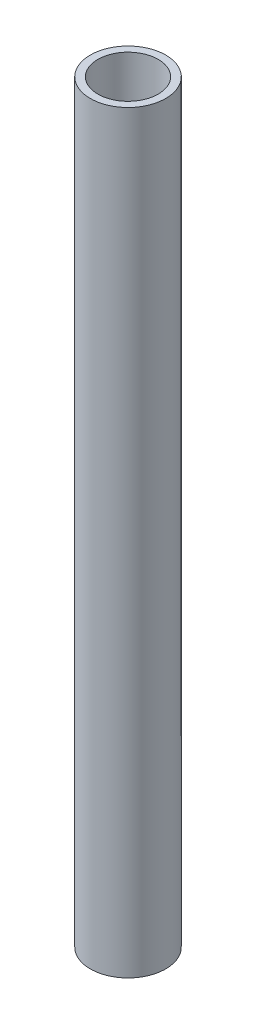
SolidWorks part; units mm, degrees
material "Q235B"
ref_plane "Front Plane" through (0, 0, 0) normal (0, 0, 1) x (1, 0, 0)
ref_plane "Top Plane" through (0, 0, 0) normal (0, 1, 0) x (1, 0, 0)
ref_plane "Right Plane" through (0, 0, 0) normal (1, 0, 0) x (0, 0, -1)
sketch "Sketch1" plane through (0, 0, 0) normal (0, 0, 1) x (1, 0, 0)
  line L0 (0, 0) -> (0, 200)
  dimension "D1" = 200
other "GB/T 6728-2002 round tube 20 × 2(1)"
ref_plane "Plane1" through (0, 0, 0) normal (0, 1, 0) x (-1, 0, 0)
sketch "Sketch11" plane through (0, 0, 0) normal (0, 1, 0) x (-1, 0, 0)
  circle A0 centre (0, 0) radius 8
  circle A1 centre (0, 0) radius 10
  point P3 (0, 0)
  dimension "Out_dia" = 20
  dimension "D1" = 2
